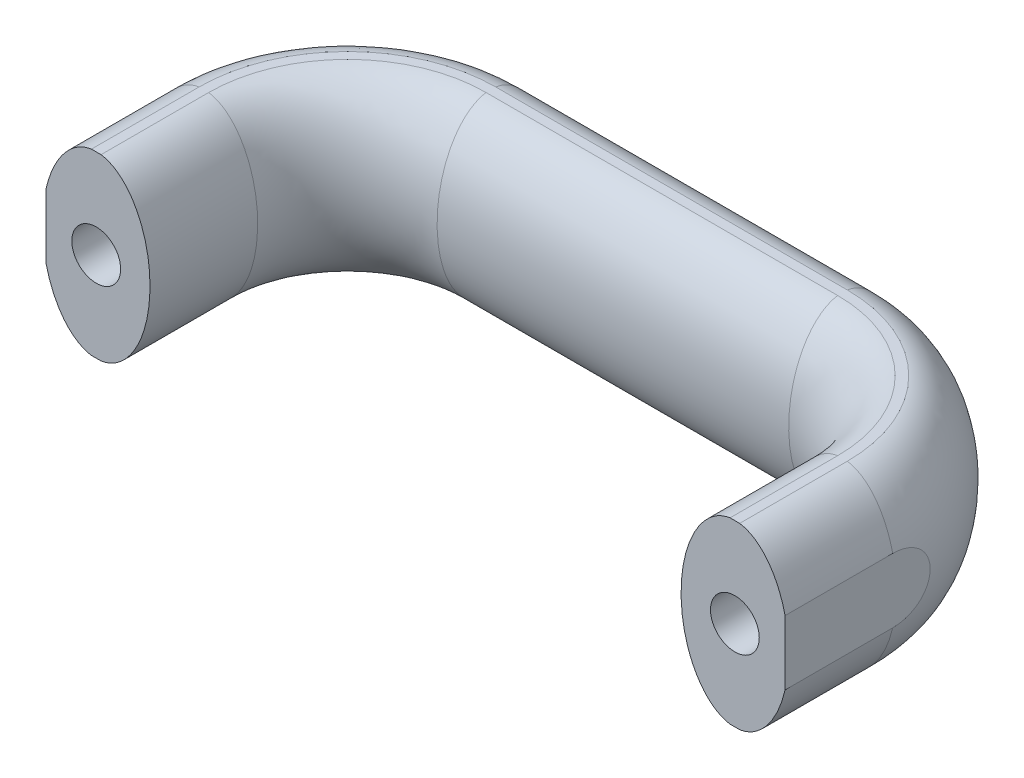
from build123d import *

# Parameters (mm, degrees)
SKETCH2_RX              = 12.5
SKETCH2_RY              = 7.5
M8_TAPPED_HOLE1_D       = 6.8
M8_TAPPED_HOLE1_DEPTH   = 19.75
M8_TAPPED_HOLE1_TIP     = 2.042926105
SKETCH6_W               = 123
SKETCH6_H               = 44.9
SKETCH6_W_2             = 103
SKETCH6_H_2             = 24.9
CUT_EXTRUDE_THIN1_DEPTH = 107.18262584


with BuildPart() as part:
    # Sweep1: sweep along a path in Sketch3
    with BuildLine(Plane(origin=(0, 0, 0), x_dir=(1, 0, 0), z_dir=(0, 1, 0))) as sweep1_path:
        Line((0, 0), (0, 15))
        ThreePointArc((0, 15), (5.857864376, 29.142135624), (20, 35))
        Line((20, 35), (69, 35))
        ThreePointArc((69, 35), (83.142135624, 29.142135624), (89, 15))
        Line((89, 15), (89, 0))
    # Sketch2 → Sweep1 (sweep)
    with BuildSketch(Plane.XY):
        with Locations(Location((0, 0), (0, 0, 90))):
            Ellipse(SKETCH2_RX, SKETCH2_RY)
    sweep(path=sweep1_path.line)

    # M8 Tapped Hole1
    with Locations(Plane.XY):
        with Locations((0, 0), (89, 0)):
            Hole(M8_TAPPED_HOLE1_D / 2, depth=M8_TAPPED_HOLE1_DEPTH)
            with Locations((0, 0, -(M8_TAPPED_HOLE1_DEPTH + M8_TAPPED_HOLE1_TIP / 2))):  # 118° drill point
                Cone(0, M8_TAPPED_HOLE1_D / 2, M8_TAPPED_HOLE1_TIP, mode=Mode.SUBTRACT)

    # Sketch6 → Cut-Extrude-Thin1 (cut, through all)
    with BuildSketch(Plane.XY):
        with Locations((44.5, 0)):
            Rectangle(SKETCH6_W, SKETCH6_H)
        with Locations((44.5, 0)):
            Rectangle(SKETCH6_W_2, SKETCH6_H_2, mode=Mode.SUBTRACT)
    extrude(amount=-CUT_EXTRUDE_THIN1_DEPTH, mode=Mode.SUBTRACT)


solid = part.part
